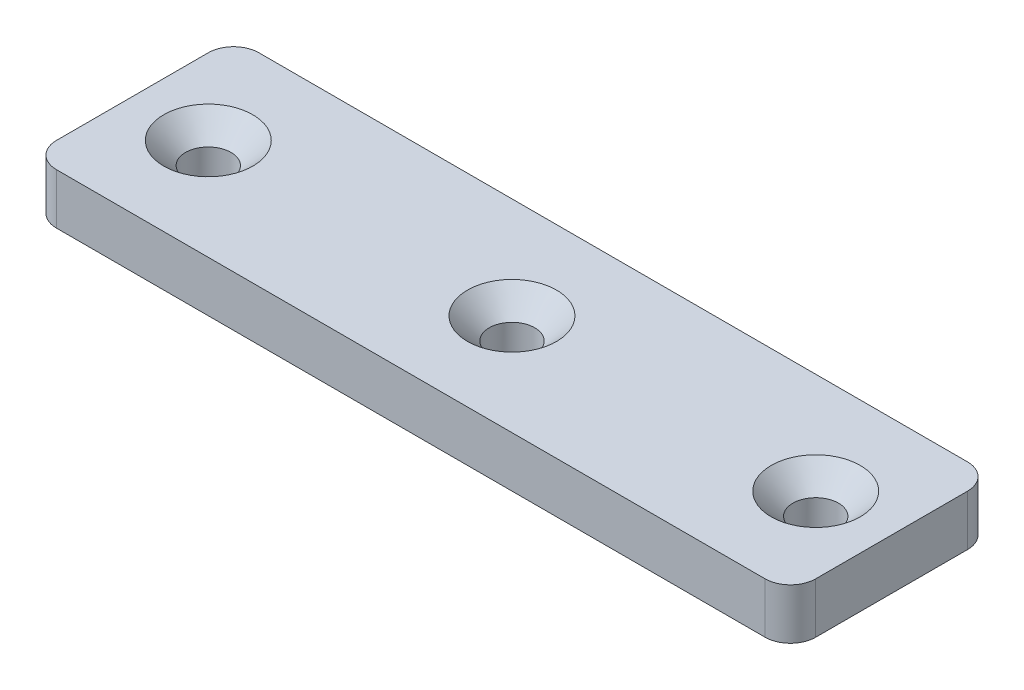
SolidWorks part; units mm, degrees
ref_plane "Front Plane" through (0, 0, 0) normal (0, 0, 1) x (1, 0, 0)
ref_plane "Top Plane" through (0, 0, 0) normal (0, 1, 0) x (1, 0, 0)
ref_plane "Right Plane" through (0, 0, 0) normal (1, 0, 0) x (0, 0, -1)
sketch "Sketch1" plane through (0, 0, 0) normal (0, 1, 0) x (1, 0, 0)
  line L1 (0, 0) -> (150, 0)
  line L2 (0, 0) -> (0, 40)
  line L3 (0, 40) -> (150, 40)
  line L4 (150, 0) -> (150, 40)
  dimension "D1" = 150
  dimension "D2" = 40
extrude "Boss-Extrude1" add sketch "Sketch1" along normal blind 10
fillet "Fillet1" radius 5 4 edges at (0, 5, -40) (150, 5, -40) (150, 5, 0) (0, 5, 0)
sketch "Sketch3" plane through (0, 0, 0) normal (0, -1, 0) x (1, 0, 0)
  line L0 (5, 0) -> (145, 0) construction
  line L1 (0, -35) -> (0, -5) construction
  circle A0 centre (16, -19) radius 11
  circle A1 centre (16, -19) radius 9
  dimension "D1" = 22
  dimension "D2" = 18
  dimension "D3" = 19
  dimension "D4" = 16
extrude "Cut-Extrude2" [suppressed] cut sketch "Sketch3" against normal blind 2
pattern_linear "LPattern1" [suppressed] count 5 spacing 13
pattern_linear "LPattern2" [suppressed] count 7 spacing 28
hole_wizard "Socket Button Head Screw Hole1" positions "Sketch4" profile "Sketch5" countersink size "M8" standard "GB"
sketch "Sketch4" plane through (0, 10, 0) normal (0, 1, 0) x (1, 0, 0)
  line L0 (75, 0) -> (75, 20) construction
  line L1 (5, 0) -> (145, 0) construction
  line L3 (0, 20) -> (15, 20) construction
  line L4 (0, 35) -> (0, 5) construction
  point P0 (75, 20)
  point P2 (15, 20)
  point P4 (135, 20)
  dimension "D1" = 120
sketch "Sketch5" plane through (75, 10, -20) normal (1, 0, 0) x (0, 0, 1)
  line L0 (0, 0) -> (0, 22.4539)
  line L1 (0, 22.4539) -> (4.5, 19.75)
  line L2 (4.5, 19.75) -> (4.5, 4.3)
  line L3 (4.5, 4.3) -> (8.8, 0)
  line L5 (8.8, 0) -> (0, 0)
  line L6 (-4.5, 4.3) -> (-8.8, 0) construction
  line L10 (0, 22.4539) -> (-4.5, 19.75) construction
  line L11 (0, -6.35) -> (0, 107.95) construction
  dimension "孔直径" = 9
  dimension "孔深度" = 19.75
  dimension "近端锥形沉头孔直径" = 17.6
  dimension "近端锥形沉头孔角度" = 90
  dimension "导头角度" = 118
